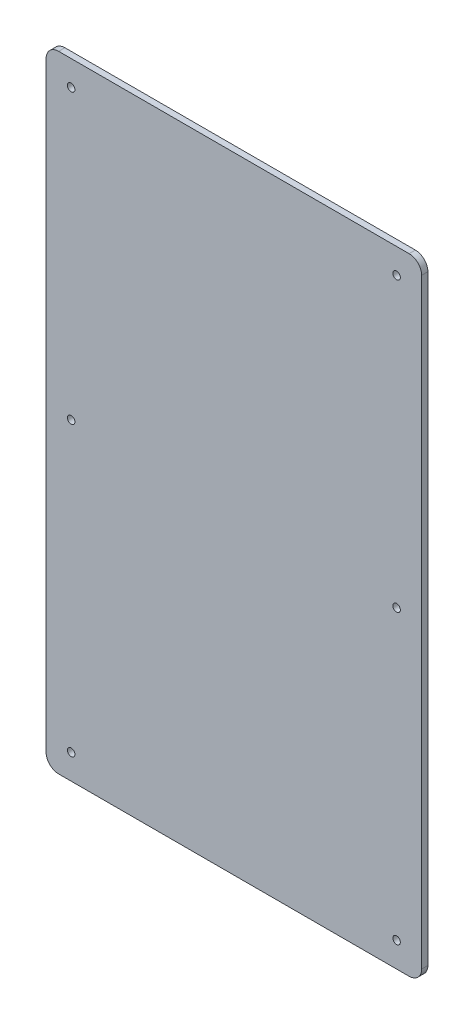
from build123d import *

# Parameters (mm, degrees)
SKETCH_1_W                = 300
SKETCH_1_H                = 500
EXTRUDE_1_DEPTH           = 5
HOLE_WIZARD_6_0_6_1_D     = 6
HOLE_WIZARD_6_0_6_1_DEPTH = 27.75
HOLE_WIZARD_6_0_6_1_TIP   = 1.802581857
FILLET_1_R                = 10


with BuildPart() as part:
    # 草图1 → 凸台-拉伸1 (new body)
    with BuildSketch(Plane.XY):
        Rectangle(SKETCH_1_W, SKETCH_1_H)
    extrude(amount=EXTRUDE_1_DEPTH)

    # Ø6.0 (6) 直径孔1
    with Locations(Plane.XY.offset(5)):
        with Locations((-130, 230), (130, 230), (130, -230), (-130, -230), (-130, 0), (130, 0)):
            Hole(HOLE_WIZARD_6_0_6_1_D / 2, depth=HOLE_WIZARD_6_0_6_1_DEPTH)
            with Locations((0, 0, -(HOLE_WIZARD_6_0_6_1_DEPTH + HOLE_WIZARD_6_0_6_1_TIP / 2))):  # 118° drill point
                Cone(0, HOLE_WIZARD_6_0_6_1_D / 2, HOLE_WIZARD_6_0_6_1_TIP, mode=Mode.SUBTRACT)

    # 圆角1
    fillet_1_edges = [part.edges().sort_by_distance(p)[0] for p in [
        (150, -250, 2.5),
        (-150, -250, 2.5),
        (-150, 250, 2.5),
        (150, 250, 2.5),
    ]]
    fillet(fillet_1_edges, radius=FILLET_1_R)


solid = part.part
